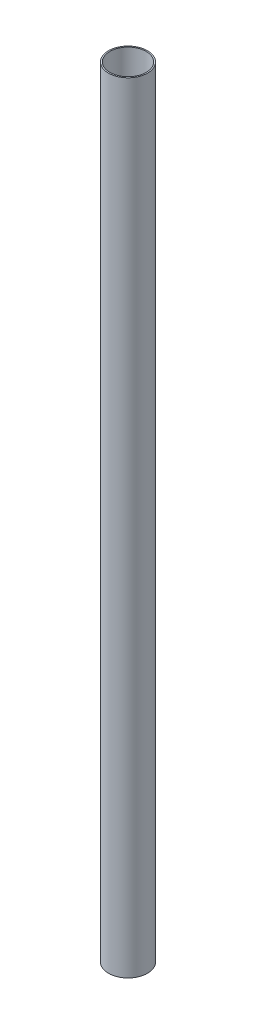
from build123d import *

# Parameters (mm, degrees)
SWEEP_THIN1_PROFILE_R   = 15
SWEEP_THIN1_PROFILE_R_2 = 14


with BuildPart() as part:
    # Sweep-Thin1: sweep along a path in Sketch1
    with BuildLine(Plane.XY) as sweep_thin1_path:
        Line((0, 0), (0, 600))
    # Sweep-Thin1 profile (on start of the path) → Sweep-Thin1 (sweep)
    with BuildSketch(Plane.ZX):
        Circle(SWEEP_THIN1_PROFILE_R)
        Circle(SWEEP_THIN1_PROFILE_R_2, mode=Mode.SUBTRACT)
    sweep(path=sweep_thin1_path.line)


solid = part.part
